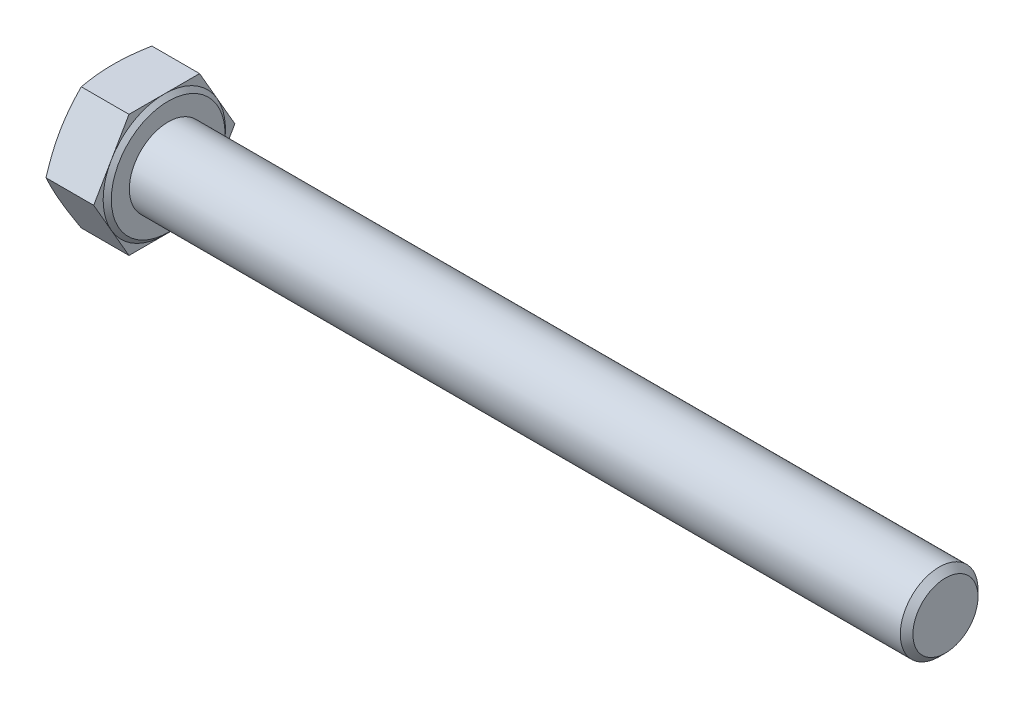
from build123d import *

# Parameters (mm, degrees)
BASEHEAD_DEPTH = 6.58
SKETCH3_R      = 5
BASEBODY_DEPTH = 100
CHAMFER1_SIZE  = 0.812


with BuildPart() as part:
    # Sketch-BaseHead → BaseHead (new body)
    with BuildSketch(Plane(origin=(0, 0, 0), x_dir=(0, 0, -1), z_dir=(1, 0, 0))):
        Polygon((9.081719734, 0), (4.540859867, 7.865), (-4.540859867, 7.865), (-9.081719734, 0), (-4.540859867, -7.865), (4.540859867, -7.865), align=None)
    extrude(amount=BASEHEAD_DEPTH)

    # Sketch4 → HeadChamfer (revolve, cut)
    with BuildSketch(Plane(origin=(-0.264637255, 0, 5.916896391), x_dir=(0, 0, -1), z_dir=(0, 1, 0))):
        Polygon((14.998616125, -0.264637255), (13.781896391, -0.264637255), (14.998616125, -0.707487022), align=None)
    revolve(axis=Axis((-4.001564945, 0, 0), (1, 0, 0)), mode=Mode.SUBTRACT)

    # Sketch1 → Revolve1 (revolve)
    with BuildSketch(Plane.XY, mode=Mode.PRIVATE) as revolve1_sk:
        Polygon((6.58, 0), (7.08, 0), (7.08, -7.315), (6.58, -7.865), align=None)
    revolve(revolve1_sk.sketch.rotate(Axis((-4.001564945, 0, 0), (1, 0, 0)), 270), axis=Axis((-4.001564945, 0, 0), (1, 0, 0)))

    # Sketch3 → BaseBody (add)
    with BuildSketch(Plane(origin=(7.08, 0, 0), x_dir=(0, 0, -1), z_dir=(1, 0, 0))):
        Circle(SKETCH3_R)
    extrude(amount=BASEBODY_DEPTH)

    # Chamfer1
    chamfer1_edges = [part.edges().sort_by_distance(p)[0] for p in [
        (107.08, 0, 5),
    ]]
    chamfer(chamfer1_edges, length=CHAMFER1_SIZE)


solid = part.part
